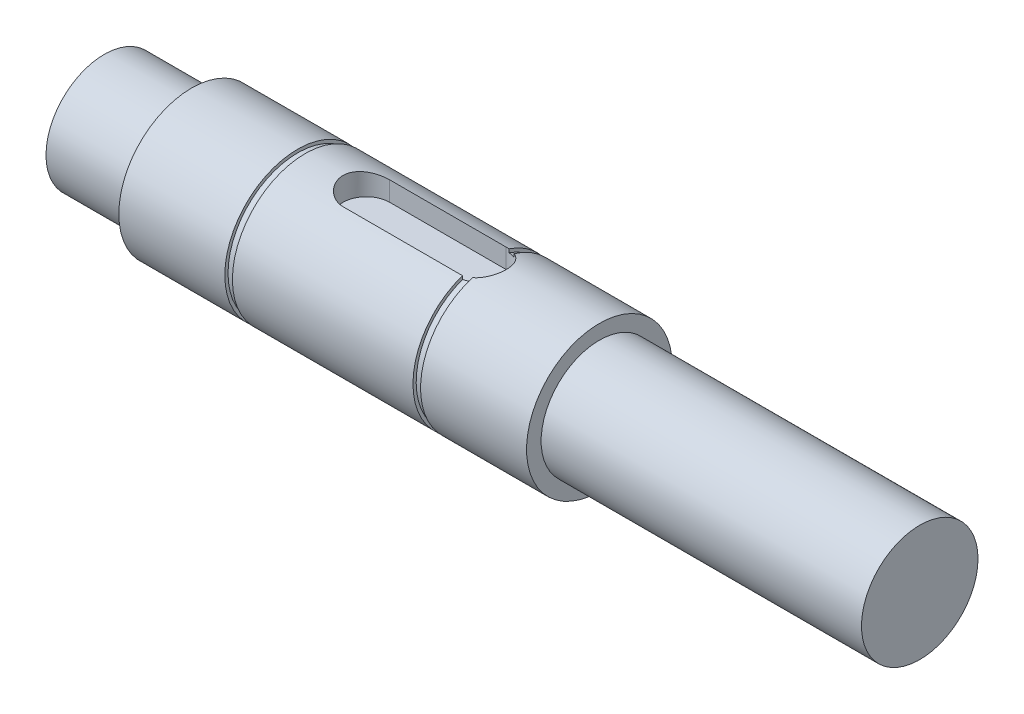
from build123d import *

# Parameters (mm, degrees)
SKETCH_1_R          = 12.5
EXTRUDE_1_DEPTH     = 35
SKETCH_3_R          = 10
EXTRUDE_3_DEPTH     = 55
SKETCH_4_W          = 1.3
SKETCH_4_H          = 0.55
CUT_EXTRUDE_1_DEPTH = 94.259047818
EXTRUDE_START       = 15
SKETCH_6_R          = 10
EXTRUDE_4_DEPTH     = 15


with BuildPart() as part:
    # 草图1 → 凸台-拉伸1 (new, symmetric)
    with BuildSketch(Plane(origin=(0, 0, 0), x_dir=(0, 0, -1), z_dir=(1, 0, 0))):
        Circle(SKETCH_1_R)
    extrude(amount=EXTRUDE_1_DEPTH, both=True)

    # 草图3 → 凸台-拉伸3 (add)
    with BuildSketch(Plane(origin=(35, 0, 0), x_dir=(0, 0, -1), z_dir=(1, 0, 0))):
        Circle(SKETCH_3_R)
    extrude(amount=EXTRUDE_3_DEPTH)

    # 草图4 → 切除-旋转1 (revolve, cut)
    with BuildSketch(Plane(origin=(0, 0, 0), x_dir=(1, 0, 0), z_dir=(0, 1, 0)), mode=Mode.PRIVATE) as cut_revolve_1_sk:
        with Locations((-16.15, 12.225)):
            Rectangle(SKETCH_4_W, SKETCH_4_H)
        with Locations((16.15, 12.225)):
            Rectangle(SKETCH_4_W, SKETCH_4_H)
    revolve(cut_revolve_1_sk.sketch.rotate(Axis((0, 0, 0), (1, 0, 0)), 180), axis=Axis((0, 0, 0), (1, 0, 0)), mode=Mode.SUBTRACT)

    # 草图5 → 切除-拉伸1 (cut, through all)
    with BuildSketch(Plane(origin=(0, 8.5, 0), x_dir=(1, 0, 0), z_dir=(0, 1, 0))):
        with BuildLine():
            Line((-5, 4), (15, 4))
            ThreePointArc((15, 4), (19, 0), (15, -4))
            Line((15, -4), (-5, -4))
            ThreePointArc((-5, -4), (-9, 0), (-5, 4))
        make_face()
    extrude(amount=CUT_EXTRUDE_1_DEPTH, mode=Mode.SUBTRACT)

    # 草图6 → 凸台-拉伸4 (add)
    with BuildSketch(Plane.ZY.offset(35).offset(EXTRUDE_START)):
        with Locations(Location((0, 0, 0), (0, 0, 180))):
            Circle(SKETCH_6_R)
    extrude(amount=-EXTRUDE_4_DEPTH)


solid = part.part
